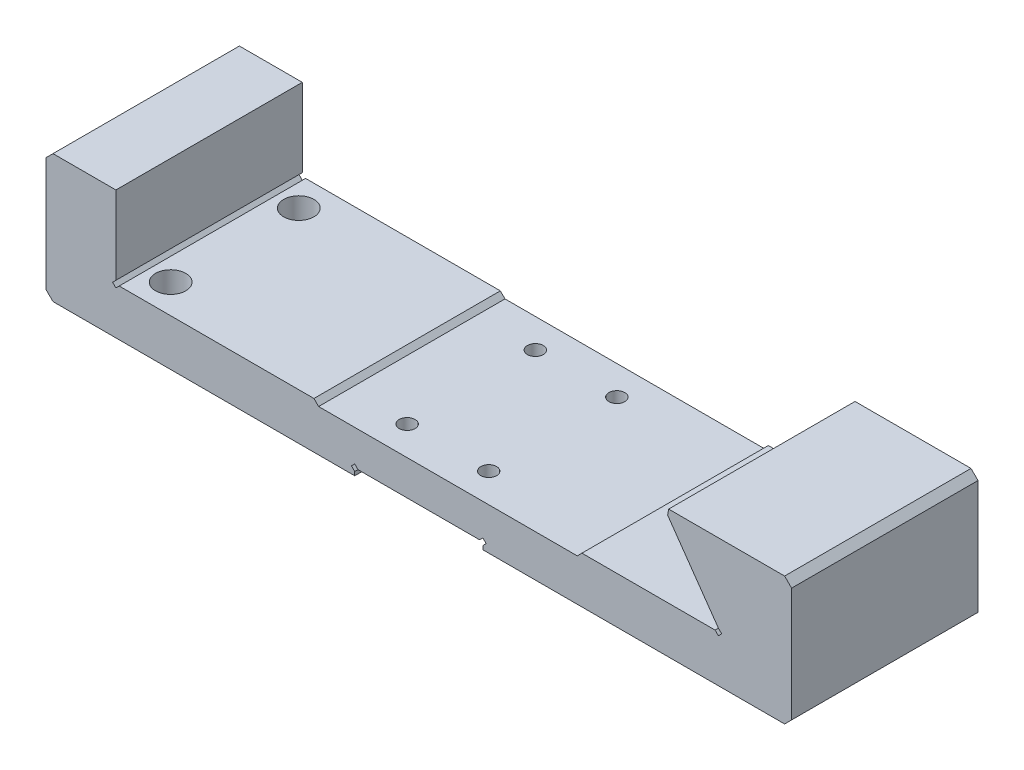
from build123d import *
from OCP.BRepFilletAPI import BRepFilletAPI_MakeChamfer

# Parameters (mm, degrees)
SKETCH1_W           = 320
SKETCH1_H           = 80
BOSS_EXTRUDE1_DEPTH = 55
CUT_EXTRUDE1_DEPTH  = 188.149672722
CUT_EXTRUDE2_DEPTH  = 188.149672722
SKETCH7_R           = 6.5
CUT_EXTRUDE3_DEPTH  = 169.597153001
CHAMFER1_SIZE       = 3
CHAMFER1_SIZE2      = 2.154045129


with BuildPart() as part:
    # Sketch1 → Boss-Extrude1 (new body)
    with BuildSketch(Plane(origin=(0, 0, 0), x_dir=(1, 0, 0), z_dir=(0, 1, 0))):
        Rectangle(SKETCH1_W, SKETCH1_H)
    extrude(amount=BOSS_EXTRUDE1_DEPTH)

    # Sketch2 → Cut-Extrude1 (cut, through all)
    with BuildSketch(Plane.XY.offset(40)):
        Polygon((105.068765597, 55), (128.585786438, 21.414213562), (130, 20), (128.585786438, 18.585786438), (127.171572875, 20), (70, 20), (68, 18), (-43, 18), (-45, 20), (-128.585786438, 20), (-130, 18.585786438), (-131.414213562, 20), (-130, 21.414213562), (-130, 55), align=None)
    extrude(amount=-CUT_EXTRUDE1_DEPTH, mode=Mode.SUBTRACT)

    # Sketch3 → Cut-Extrude2 (cut, through all)
    with BuildSketch(Plane.XY.offset(40)):
        Polygon((-26.085786438, 3), (26.085786438, 3), (27.5, 4.414213562), (28.914213562, 3), (27.5, 1.585786438), (27.5, 0), (-27.5, 0), (-27.5, 1.585786438), (-28.914213562, 3), (-27.5, 4.414213562), align=None)
    extrude(amount=-CUT_EXTRUDE2_DEPTH, mode=Mode.SUBTRACT)

    # Sketch6 → M8 Tapped Hole1 (revolve, cut)
    with BuildSketch(Plane(origin=(17.5, 3, -27.5), x_dir=(0, 0, -1), z_dir=(1, 0, 0))):
        Polygon((0, 0), (0, 21.792926105), (3.4, 19.75), (3.4, 0.625), (4.025, 0), align=None)
    m8_tapped_hole1 = revolve(axis=Axis((17.5, -3.35, -27.5), (0, 1, 0)), mode=Mode.SUBTRACT)

    # Mirror1: M8 Tapped Hole1 across plane
    add(m8_tapped_hole1.mirror(Plane(origin=(0, 0, 0), x_dir=(0, 0, 1), z_dir=(1, 0, 0))), mode=Mode.SUBTRACT)

    # Mirror2: M8 Tapped Hole1 across plane
    add(m8_tapped_hole1.mirror(Plane.XY), mode=Mode.SUBTRACT)

    # Mirror2 copy 1 sketch → Mirror2 copy 1 (revolve, cut)
    with BuildSketch(Plane(origin=(-17.5, 3, 27.5), x_dir=(0, 0, 1), z_dir=(-1, 0, 0))):
        Polygon((0, 0), (0, 21.792926105), (3.4, 19.75), (3.4, 0.625), (4.025, 0), align=None)
    revolve(axis=Axis((-17.5, -3.35, 27.5), (0, 1, 0)), mode=Mode.SUBTRACT)

    # Sketch7 → Cut-Extrude3 (cut, through all)
    with BuildSketch(Plane(origin=(0, 20, 0), x_dir=(1, 0, 0), z_dir=(0, 1, 0))):
        with Locations(Location((-119, 27.5, 0), (0, 0, 270))):
            Circle(SKETCH7_R)
        with Locations(Location((-119, -27.5, 0), (0, 0, 90))):
            Circle(SKETCH7_R)
    extrude(amount=-CUT_EXTRUDE3_DEPTH, mode=Mode.SUBTRACT)

    # Chamfer1: one chamfer whose edges measure the first distance from different faces: ONE call of the kernel's chamfer builder (chamfer() names one face for all edges)
    chamfer1_edges_1 = [part.edges().sort_by_distance(p)[0] for p in [
        (-160, 55, 0),
        (160, 55, 0),
        (-160, 0, 0),
        (160, 0, 0),
    ]]
    chamfer1_edges_2 = [part.edges().sort_by_distance(p)[0] for p in [
        (105.068765597, 55, 0),
    ]]
    chamfer1_side_2 = [part.faces().sort_by_distance(p)[0] for p in [
        (116.827276017, 38.207106781, 0),
    ]]
    chamfer1 = BRepFilletAPI_MakeChamfer(part.part.solid().wrapped)
    for e in chamfer1_edges_1:
        chamfer1.Add(CHAMFER1_SIZE, e.wrapped)
    for e in chamfer1_edges_2:
        chamfer1.Add(CHAMFER1_SIZE, CHAMFER1_SIZE2, e.wrapped, chamfer1_side_2[0].wrapped)  # the first distance lies on this face
    add(Compound.cast(chamfer1.Shape()), mode=Mode.REPLACE)


solid = part.part
